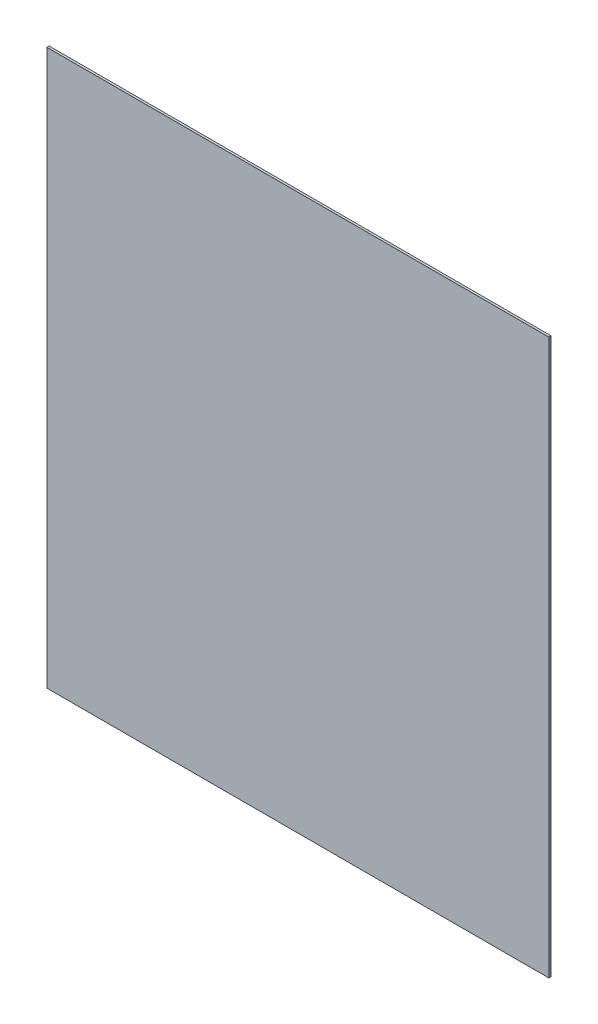
from build123d import *

# Parameters (mm, degrees)
SKETCH_1_W      = 1135
SKETCH_1_H      = 1255
EXTRUDE_1_DEPTH = 5


with BuildPart() as part:
    # 草图1 → 凸台-拉伸1 (new body)
    with BuildSketch(Plane.XY):
        Rectangle(SKETCH_1_W, SKETCH_1_H)
    extrude(amount=EXTRUDE_1_DEPTH)


solid = part.part
